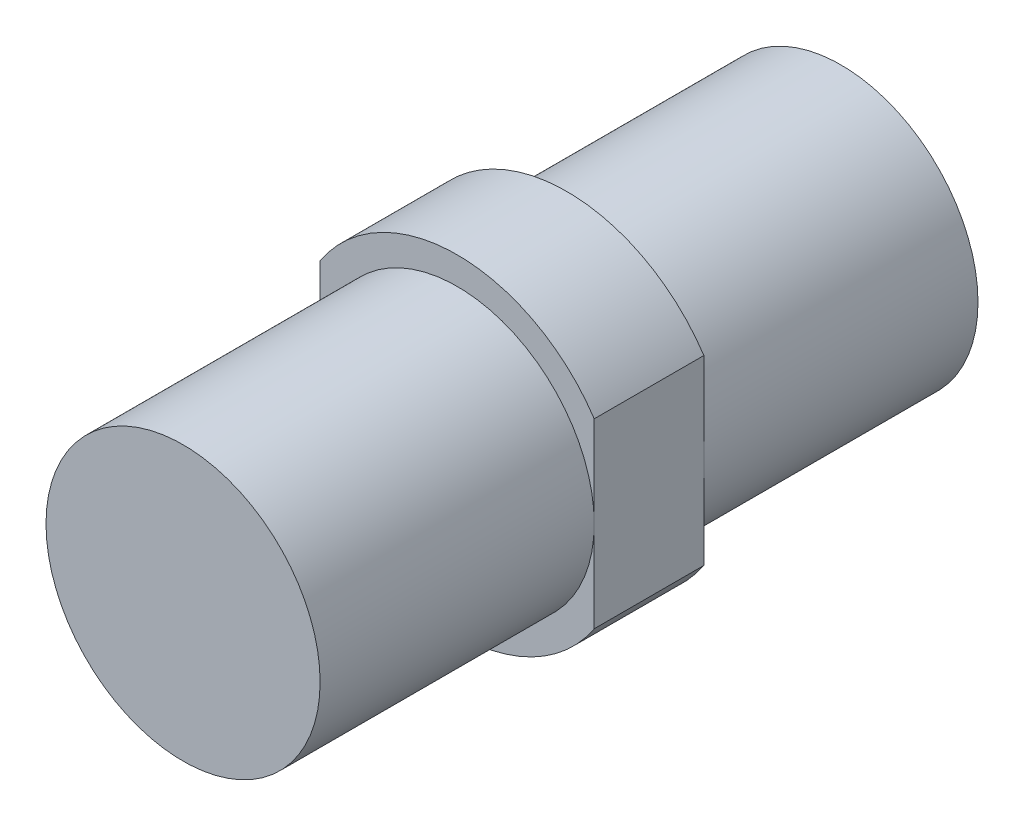
SolidWorks part; units mm, degrees
ref_plane "Front Plane" through (0, 0, 0) normal (0, 0, 1) x (1, 0, 0)
ref_plane "Top Plane" through (0, 0, 0) normal (0, 1, 0) x (1, 0, 0)
ref_plane "Right Plane" through (0, 0, 0) normal (1, 0, 0) x (0, 0, -1)
ref_plane "Plane1" through (0, 0, 4) normal (0, 0, 1) x (1, 0, 0)
sketch "Sketch1" plane through (0, 0, 4) normal (0, 0, 1) x (1, 0, 0)
  line L0 (5, -3.3166) -> (5, 3.3166)
  line L1 (-5, 3.3166) -> (-5, -3.3166)
  arc A0 (-5, -3.3166) -> (5, -3.3166) centre (0, 0) ccw
  arc A1 (5, 3.3166) -> (-5, 3.3166) centre (0, 0) ccw
extrude "Boss-Extrude1" add sketch "Sketch1" against normal blind 4
sketch "Sketch2" plane through (0, 0, 0) normal (0, 1, 0) x (1, 0, 0)
  line L0 (5, -4) -> (0, -4)
  line L1 (0, -4) -> (0, -14)
  line L2 (0, -14) -> (5, -14)
  line L3 (5, -14) -> (5, -4)
  line L4 (0, -4) -> (0, -14) construction
revolve "Revolve1" add sketch "Sketch2" angle 360 about L4
ref_plane "Plane2" through (0, 0, 0) normal (0, -1, 0) x (1, 0, 0)
sketch "Sketch3" plane through (0, 0, 0) normal (0, -1, 0) x (1, 0, 0)
  line L0 (5, 0) -> (0, 0)
  line L1 (0, 0) -> (0, -10)
  line L2 (0, -10) -> (5, -10)
  line L3 (5, -10) -> (5, 0)
  line L4 (0, 0) -> (0, -10) construction
revolve "Revolve2" add sketch "Sketch3" angle 360 about L4
